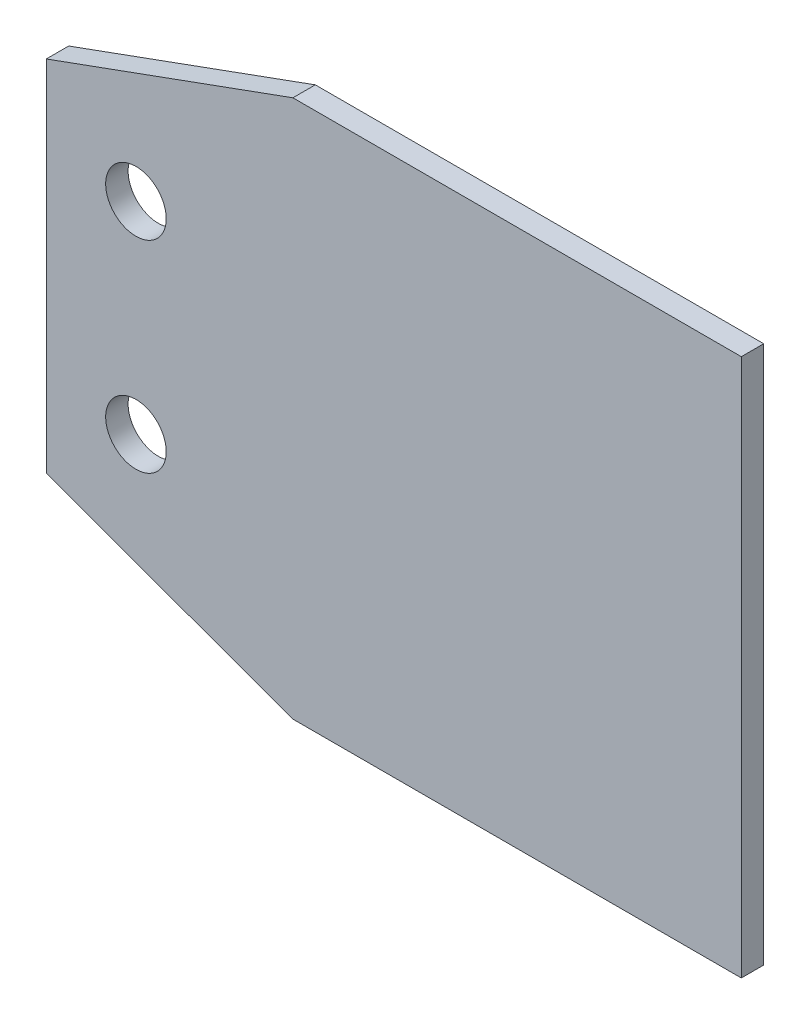
SolidWorks part; units mm, degrees
material "1023 碳钢板 (SS)"
ref_plane "前视基准面" through (0, 0, 0) normal (0, 0, 1) x (1, 0, 0)
ref_plane "上视基准面" through (0, 0, 0) normal (0, 1, 0) x (1, 0, 0)
ref_plane "右视基准面" through (0, 0, 0) normal (1, 0, 0) x (0, 0, -1)
sketch "草图1" plane through (0, 0, 0) normal (0, 0, 1) x (1, 0, 0)
  line L1 (155, 120) -> (-155, 120)
  line L2 (155, 120) -> (155, -120)
  line L3 (155, -120) -> (-155, -120)
  line L4 (-155, 120) -> (-155, -120)
  line L5 (155, 120) -> (-155, -120) construction
  line L6 (155, -120) -> (-155, 120) construction
  point P0 (0, 0)
  dimension "D1" = 310
  dimension "D2" = 240
extrude "凸台-拉伸1" add sketch "草图1" along normal blind 10
sketch "草图2" plane through (0, 0, 10) normal (0, 0, 1) x (1, 0, 0)
  line L10 (-155, 120) -> (-155, -120) construction
  line L11 (-155, -80) -> (-45, -120)
  line L12 (-155, -120) -> (155, -120) construction
  line L13 (-45, -120) -> (-155, -120)
  line L14 (-155, -120) -> (-155, -80)
  line L15 (-155, 80) -> (-45, 120)
  line L16 (155, 120) -> (-155, 120) construction
  line L17 (-45, 120) -> (-155, 120)
  line L18 (-155, 120) -> (-155, 80)
  circle A2 centre (-115, -45) radius 13.5
  circle A3 centre (-115, 45) radius 13.5
  dimension "D2" = 27
  dimension "D3" = 45
  dimension "D4" = 40
  dimension "D9" = 27
  dimension "D1" = 90
  dimension "D5" = 40
  dimension "D6" = 40
  dimension "D7" = 110
  dimension "D8" = 110
extrude "切除-拉伸1" cut sketch "草图2" against normal blind 10
